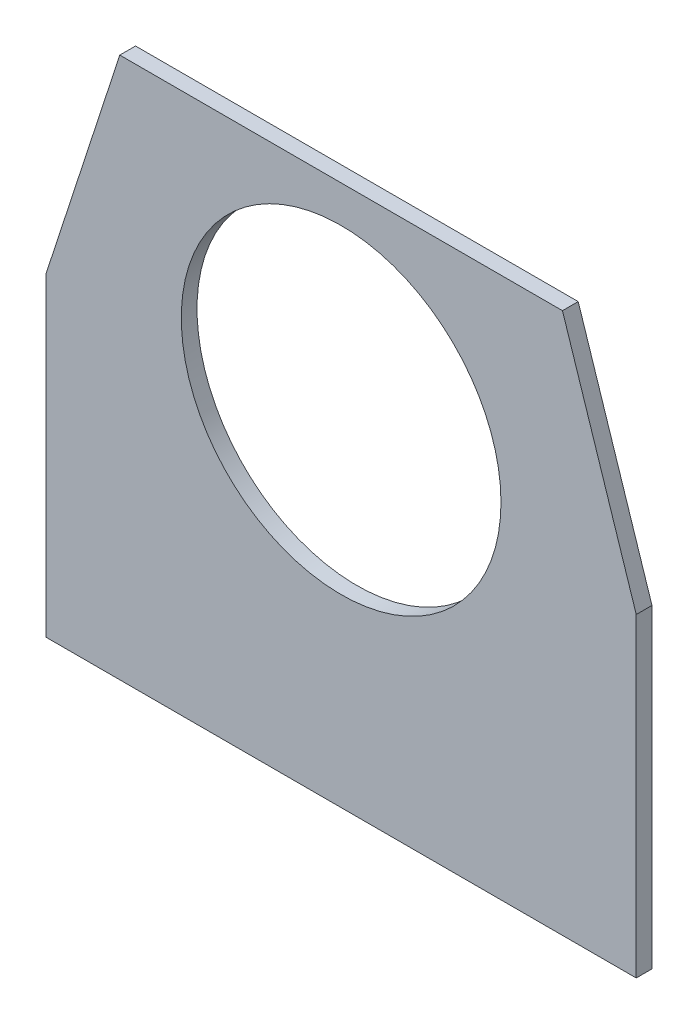
from build123d import *

# Parameters (mm, degrees)
SKETCH1_R           = 162.5
BOSS_EXTRUDE1_DEPTH = 8


with BuildPart() as part:
    # Sketch1 → Boss-Extrude1 (new, symmetric)
    with BuildSketch(Plane.XY):
        Polygon((-225, 550), (225, 550), (300, 320), (300, 0), (-300, 0), (-300, 320), align=None)
        with Locations((0, 350)):
            Circle(SKETCH1_R, mode=Mode.SUBTRACT)
    extrude(amount=BOSS_EXTRUDE1_DEPTH, both=True)


solid = part.part
